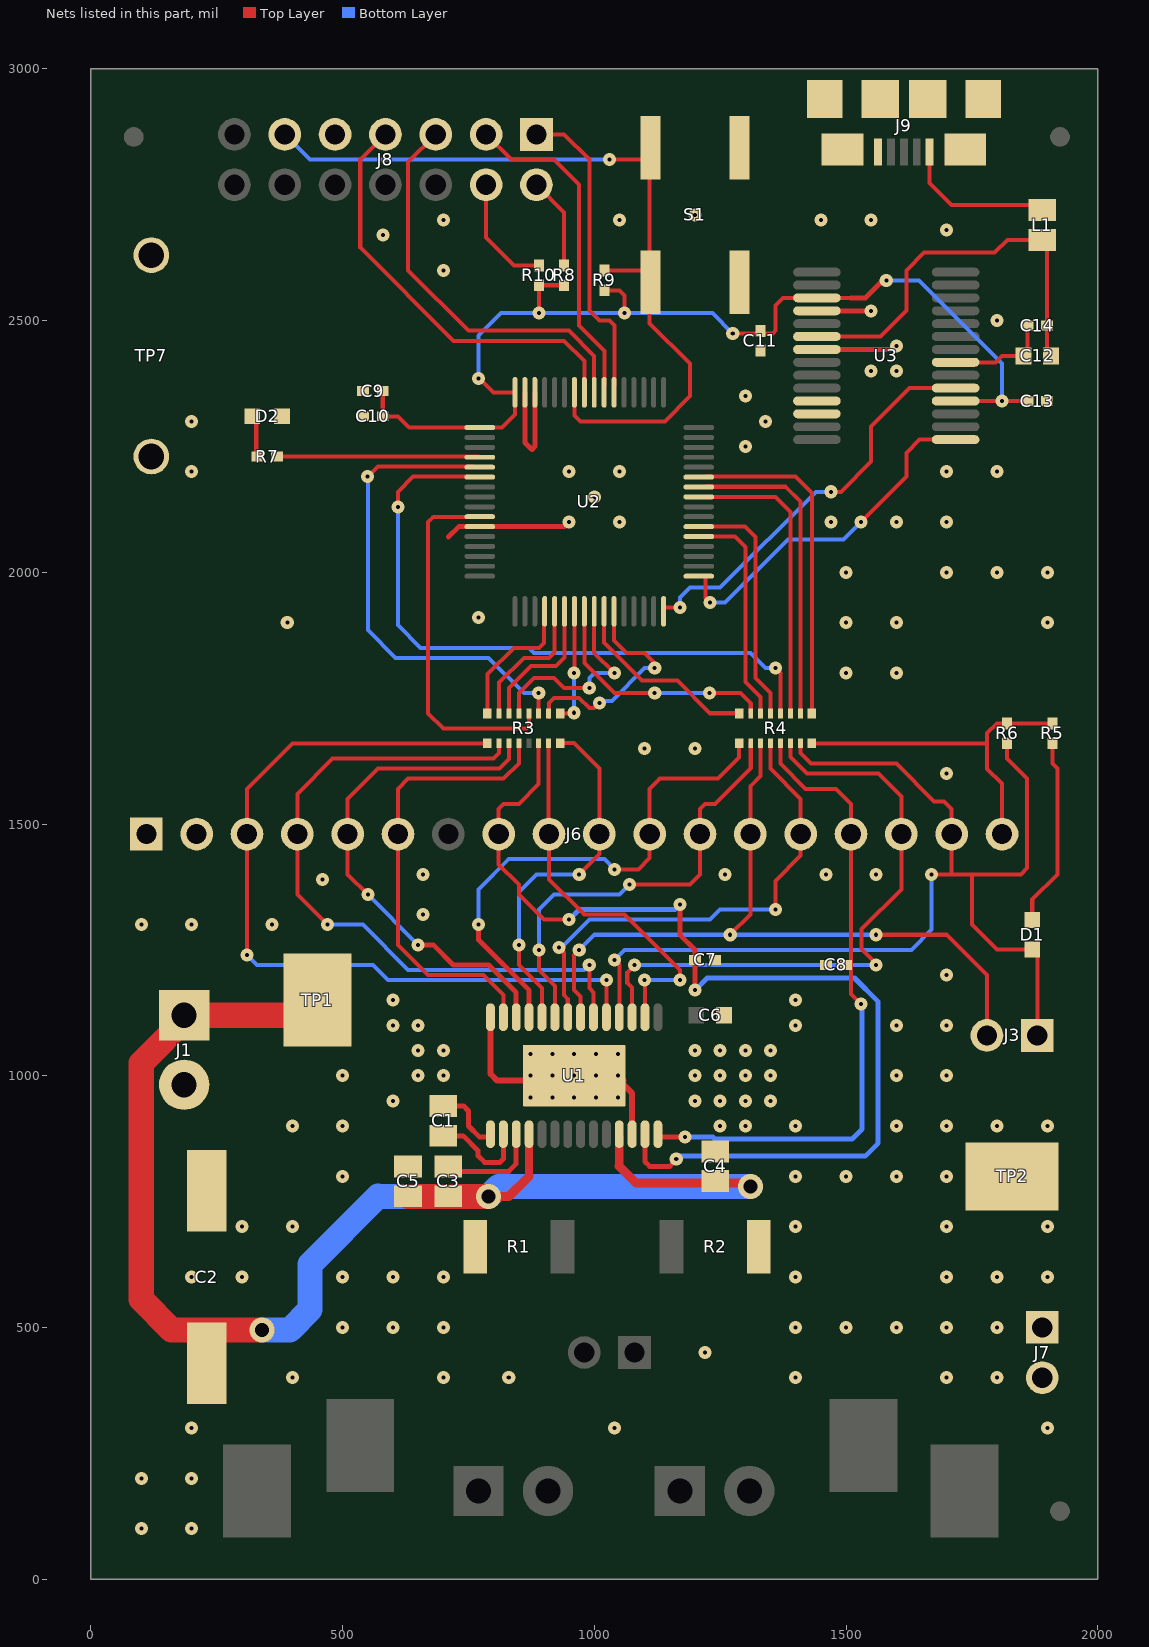
[diagram p0: the nets of this part, all layers, seen from the top]
# Altium PCB MISC86176.PcbDoc (part 2 of 2)
Units mil, origin at the board's own origin, x right, y up, seen from the top; angles counter-clockwise.
Board outline 2000 x 3000 mil, 4 copper layers (Top Layer, GND1, GND2, Bottom Layer), stack 91.4 mil thick; 53 components, 60 nets, 274 pads, 201 vias.

## Via types
v1: diameter 26, hole 8, Top Layer to Bottom Layer, tented both sides, 180 vias
v2: diameter 19.68, hole 7.87, Top Layer to Bottom Layer, 15 vias
v3: diameter 50, hole 28, Top Layer to Bottom Layer, tented both sides, 5 vias
v4: diameter 26, hole 8, Top Layer to Bottom Layer, tented top, 1 vias

## Nets (pads, with @x,y where several pads share a name; then routed paths per layer and width w, separated by ;. In a path a pad name is that pad's centre, name@x,y a point inside that pad or via, vN(x,y) a via of type N, cw(c..) or ccw(c..) an arc to the next point about the centre after c; other vN are vias at no path point) (continued)
GND: C2.2 C4.1 C5.1 C6.2 C7.2 C8.2 C9.2 C10.2 C11.2 C12.2 C13.2 C14.2 D2.2 J1.2 J6.1 J6.2 J7.1 J7.2 J8.9 J9.5 J9.6 J9.7 J9.8 J9.9 J9.10 J9.11 R1.1 R2.1 S1.1 S1.2 TP2.1 TP7.1 TP7.2 U1.12 U1.28 U1.29 U2.11 U2.62 U2.63 U3.7 U3.18 U3.21 U3.25 U3.26 | length 1423.6
  Top Layer w8: U3.7@1728.9,2417.2 1797.2,2417.2 1810,2430 C12.2@1852.44,2430 1860.31,2437.87 C14.2@1860.31,2490
  Top Layer w10: 710,2070 730.79,2090.79 U2.11@772.48,2090.79 ; U2.11@772.39,2090.7 940.7,2090.7 v1(950,2100) ; U2.63@862.05,2357.52 862.05,2257.95 876.02,2243.98 881.73,2249.69 U2.62@881.73,2357.52 ; U3.21@1430.9,2442.8 1587.2,2442.8 ; U3.18@1430.9,2519.33 U3.18@1430.9,2519.6 ; U3.18@1442.2,2519.57 1442.2,2519.33 v1(1549.33,2519.33)
  Top Layer w12: U1.28@793.66,1102.2 793.66,1003.66 807.32,990 1046.61,990 U1.29@1058.14,990 ; U1.29@1058.14,981.86 1075.16,964.84 U1.12@1075.16,883.86 U1.12@1075.16,877.8
  other v1: 100,100 200,100 100,200 200,200 200,300 1040,300 1900,300 400,400 700,400 830,400 1400,400 1700,400 1800,400 1220,450 500,500 600,500 700,500 1400,500 1500,500 1600,500 1700,500 1800,500 200,600 300,600 500,600 600,600 700,600 1400,600 1700,600 1800,600 1900,600 300,700 400,700 1400,700 1700,700 1900,700 500,800 1400,800 1500,800 1600,800 1700,800 400,900 500,900 1250,900 1300,900 1400,900 1600,900 1700,900 1800,900 1900,900 600,950 1200,950 1250,950 1300,950 1350,950 500,1000 650,1000 700,1000 1200,1000 1250,1000 1300,1000 1350,1000 1600,1000 1700,1000 650,1050 700,1050 1200,1050 1250,1050 1300,1050 1350,1050 600,1100 650,1100 1400,1100 1600,1100 1700,1100 600,1150 1400,1150 1700,1200 100,1300 200,1300 360,1300 660,1320 460,1390 660,1400 1260,1400 1460,1400 1560,1400 1700,1600 1100,1650 1200,1650 1500,1800 1600,1800 390,1900 1500,1900 1600,1900 1900,1900 770,1910 1500,2000 1700,2000 1800,2000 1900,2000 1050,2100 1470,2100 1600,2100 1700,2100 1000,2150 200,2200 950,2200 1050,2200 1700,2200 1800,2200 1300,2250 200,2300 1340,2300 1300,2350 1550,2400 1600,2400 1600,2450 1800,2500 700,2600 580,2670 1700,2680 700,2700 1050,2700 1450,2700 1550,2700 1200,2710
  other v2: 873.39,956.69 916.69,956.69 960,956.69 1003.31,956.69 1046.61,956.69 873.39,1000 916.69,1000 960,1000 1003.31,1000 1046.61,1000 873.39,1043.31 916.69,1043.31 960,1043.31 1003.31,1043.31 1046.61,1043.31
GPIO_V3P3: J6.18 R4.8 R5.2 R6.2 | length 681.8
  Top Layer w8: R4.8@1438.5,1660 1780,1660 ; J6.18@1810,1490 1810,1580 1780.31,1609.69 1780.31,1680.31 1799.69,1699.69 R6.2@1820,1699.69 R5.2@1910,1699.69
MSP_8XV3P3: R3.12 U2.10 | length 712
  Top Layer w8: U2.10@758.9,2110 680,2110 670,2100 670,1720 700,1690 865,1690 869.84,1694.84 R3.12@869.84,1719.53
MSP_ADEC_AVREF: R3.11 U2.5 | length 954.4
  Top Layer w8: v1@550,2190 570,2210 U2.5@758.9,2210 ; R3.11@889.53,1719.53 v1(889.53,1760)
  Bottom Layer w8: v1@550,2190 550,1885 605,1830 790,1830 860,1760 v1(889.53,1760) v1@890,1760
  other v1: 549.53,2190
MSP_DECAY0_ADECAY: R3.15 U2.21 | length 282.4
  Top Layer w8: R3.15@810.79,1721.5 810.79,1780.79 860,1830 867.55,1830 867.62,1830.07 910,1830.07 920.93,1841 921,1841 U2.21@921,1929
MSP_DECAY1_BDECAY: R3.16 U2.20 | length 286.3
  Top Layer w8: R3.16@787.66,1719.53 787.66,1797.66 840,1850 890,1850 900,1860 U2.20@900,1930
MSP_DIR_PHB_BIN1: R4.13 U2.38 | length 460.6
  Top Layer w8: U2.38@1220.9,2090.7 1299.3,2090.7 1320,2070 1320,1790 1350.16,1759.84 1350.16,1729.53
MSP_ENABLE_ENB_BIN2: R4.14 U2.37 | length 420.9
  Top Layer w8: U2.37@1220.9,2071 1279,2071 1300,2050 1300,1782.34 1330.47,1751.87 1330.47,1729.53
MSP_GPIO_V3P3: R4.9 U2.43 | length 653
  Top Layer w8: U2.43@1220.9,2190 1400,2190 1432.34,2157.66 1432.34,1729.53
MSP_NFAULT: R4.10 U2.42 | length 611.7
  Top Layer w8: U2.42@1220.9,2170 1380,2170 1409.21,2140.79 1409.21,1729.53
MSP_NSLEEP: R4.11 U2.41 | length 572.9
  Top Layer w8: U2.41@1220,2150 1360,2150 1390,2120 1390,1729.53
MSP_STEP_ENA_AIN2: R4.15 U2.24 | length 472.9
  Top Layer w8: U2.24@980.1,1909 980.1,1819.9 1040,1760 v1(1120,1760) ; v1(1229,1760) 1290,1760 1310.79,1739.21 R4.15@1310.79,1719.53
  Bottom Layer w8: v1(1120,1760) v1(1229,1760)
MSP_TOFF: R3.10 U2.27 | length 436.6
  Top Layer w8: R3.10@910,1712.5 910,1740 920,1750 970,1750 990,1730 1000,1730 v1(1010,1740) ; U2.27@1039.2,1909 1039.2,1864.8 1064,1840 1100,1840 1120,1820 v1(1120,1810)
  Bottom Layer w8: v1(1010,1740) 1014.8,1744.8 1034.8,1744.8 1100,1810 v1(1120,1810)
MSP_TRQ0: R3.13 U2.25 | length 400.9
  Top Layer w8: R3.13@850.16,1719.53 850.16,1760.16 880,1790 920,1790 940,1770 v1(990,1770) ; U2.25@999.8,1909 999.8,1840.2 v1(1040,1800)
  Bottom Layer w8: v1(990,1770) 990,1790 1000,1800 v1(1040,1800)
MSP_TRQ1: R3.14 U2.22 | length 284.4
  Top Layer w8: R3.14@830.47,1719.53 830.47,1770.47 874.2,1814.2 924.2,1814.2 940.7,1830.7 U2.22@940.7,1929
MSP_USM0_ADEC_PARA: R4.16 U2.26 | length 374.9
  Top Layer w8: U2.26@1019.5,1909 1019.5,1860.5 1095.13,1784.87 1165.23,1784.87 1230,1720 R4.16@1287.66,1720
MSP_USM1_PHA_AIN1: R3.9 U2.23 | length 215.4
  Top Layer w8: R3.9@932.34,1719.53 v1@959.53,1719.53 ; v1(960,1800) 960.4,1800.4 U2.23@960.4,1909
  Bottom Layer w8: v1(960,1721) v1(960,1800)
MSP_VREF_BVREF: R4.12 U2.6 | length 1287.2
  Top Layer w8: v1(610,2130) 610,2160 640,2190 U2.6@750,2190 ; v1(1359.92,1810.08) 1369.84,1800.16 1369.84,1729.53
  Bottom Layer w8: v1(610,2130) 610,1895 655,1850 870,1850 880,1840 1310.16,1840 1340.08,1810.08 v1(1359.92,1810.08)
NetC1_1: C1.1 U1.1 | length 137.2
  Top Layer w10: C1.1@700,939.53 700.47,940 740,940 750,930 750,900 772.2,877.8 U1.1@793.66,877.8
NetC1_2: C1.2 U1.2 | length 192.9
  Top Layer w10: C1.2@700,880.47 739.53,880.47 769.05,850.95 769.05,840.95 782.12,827.88 812.65,827.88 819.25,834.49 U1.2@819.25,877.8
NetD1_1: D1.1 R5.1 | length 375.6
  Top Layer w8: D1.1@1870,1309.53 1870,1350 1920,1400 1920,1610 1910,1620 R5.1@1910,1660.32
NetD2_1: D2.1 R7.1 | length 79
  Top Layer w8: R7.1@328.35,2230 D2.1@328.35,2308.99
NetJ8_2: J8.2 R8.2 | length 210.1
  Top Layer w8: J8.2@910,2770 J8.2@885,2770 940,2715 R8.2@940,2609.69 R8.2@940,2607.72
NetJ8_4: J8.4 R10.2 | length 232.5
  Top Layer w8: J8.4@785,2770 785,2665 840,2610 R10.2@889.69,2610
NFAULT: D1.2 J3.1 J6.17 R4.7 R6.1 U1.18 | length 2265.3
  Top Layer w8: v1(1040,1230) 1049.57,1220.43 U1.18@1049.57,1116.14 U1.18@1049.57,1102.2 ; R4.7@1409.21,1660.47 1409.21,1640.79 1430,1620 1600,1620 1675,1545 1695,1545 1710,1530 J6.17@1710,1480 1710,1400 ; v1(1670,1400) 1710,1400 ; R6.1@1820,1662.28 R6.1@1820,1660.32 1819.68,1630.32 1860,1590 1860,1412.2 1847.8,1400 1750,1400 ; D1.2@1870,1250.47 1799.53,1250.47 1750,1300 1750,1400 ; J3.1@1880,1080 D1.2@1880,1250 ; 1710,1400 1750,1400
  Bottom Layer w8: v1(1040,1230) 1060,1250 1630,1250 1670,1290 v1(1670,1400)
NSLEEP: J6.16 R4.6 U1.17 | length 1257.8
  Top Layer w8: U1.17@1075.16,1102.2 U1.17@1075.16,1116.14 1075.16,1174.84 1065.44,1184.56 1065.44,1205.44 v1(1080,1220) ; R4.6@1389.53,1660.47 1389.53,1632.82 1422.34,1600 1565,1600 1610,1555 J6.16@1610,1480 1610,1370 1531.22,1291.22 1531.22,1251.22 1560,1222.45 v1(1560,1220)
  Bottom Layer w8: v1@1090,1220 v1(1560,1220)
PIN13: C7.1 J6.8 R3.6 U1.13 | length 2093
  Top Layer w8: R3.6@889.53,1660.47 889.53,1579.53 850,1540 820,1540 810,1530 J6.8@810,1480 810,1420 850,1380 850,1360 900,1310 v1(950,1310)
  Top Layer w10: U1.13@1100.75,857.8 1100.75,829.25 1110,820 1150,820 1162.76,832.76 v1(1162.76,834.49) ; v1(1170,1340) 1170,1280 1200.32,1249.68 C7.1@1200.32,1230 v1(1200.32,1170)
  Bottom Layer w10: v1(950,1310) 970,1330 1160,1330 v1(1170,1340) ; v1(1162.76,834.49) 1168.27,840 1538,840 1564,866 1564,1147 1517,1194 1224.32,1194 v1(1200.32,1170)
PIN14: C8.1 J6.15 R4.5 U1.14 | length 1285.5
  Top Layer w8: R4.5@1369.84,1660.47 1369.84,1620.16 1420,1570 1480,1570 1510,1540 J6.15@1510,1480 1510,1162 v1(1530,1142)
  Top Layer w10: U1.14@1126.34,877.8 v1(1180,877.8)
  Bottom Layer w10: v1@1183.6,874.2 v1(1180,877.8) 1235.61,877.8 1239.28,874.13 1512.13,874.13 1532,894 v1@1532,1139
PIN19: J6.3 R3.1 U1.19 | length 1649.6
  Top Layer w8: v1(310,1240) J6.3@310,1480 310,1570 400,1660 R3.1@787.66,1660 ; U1.19@1023.98,1120 v1(1023.98,1190)
  Bottom Layer w8: v1(310,1240) 330,1220 560,1220 590,1190 v1(1023.98,1190)
PIN20: J6.4 R3.2 U1.20 | length 1404.4
  Top Layer w8: v1(470,1300) 410,1360 J6.4@410,1480 410,1560 480,1630 800,1630 810.79,1640.79 R3.2@810.79,1660.47 ; v1(990,1220) 990,1173.98 998.39,1165.59 998.39,1121.61 U1.20@1000,1120
  Bottom Layer w8: v1(470,1300) 540,1300 630,1210 980,1210 v1(990,1220)
PIN21: J3.2 J6.13 R4.3 U1.21 | length 1520.5
  Top Layer w8: v1(970,1250) 960,1240 960,1170 972.8,1157.2 U1.21@972.8,1120 ; v1(1270,1280) 1310,1320 J6.13@1310,1480 1310,1575 1330.47,1595.47 R4.3@1330.47,1660.47 ; v1(1560,1280) 1700,1280 1780,1200 J3.2@1780,1080
  Bottom Layer w8: v1(970,1250) 1000,1280 v1(1270,1280) v1(1560,1280)
PIN22: J6.14 R4.4 U1.22 | length 979.2
  Top Layer w8: v1(930,1255) 940,1245 940,1160 947.2,1152.8 U1.22@947.2,1120 ; R4.4@1350.16,1660.47 1350.16,1609.84 1410,1550 J6.14@1410,1480 1410,1437 1360,1387 v1(1360,1330)
  Bottom Layer w8: v1(930,1255) 935,1255 990,1310 1230,1310 1250,1330 v1(1360,1330)
PIN23: J6.12 R4.2 U1.23 | length 876
  Top Layer w8: v1(890,1250) 890,1210 921.61,1178.39 U1.23@921.61,1120 ; v1(1070,1380) 1190,1380 1210,1400 J6.12@1210,1480 1210,1530 1220,1540 1240,1540 1310.79,1610.79 R4.2@1310.79,1660.47
  Bottom Layer w8: v1@890,1260 890,1330 920,1360 1050,1360 v1(1070,1380)
PIN24: J6.10 R3.8 U1.24 | length 723.7
  Top Layer w8: v1(850,1260) 850,1220 896.02,1173.98 U1.24@896.02,1120 ; R3.8@932.34,1660.47 959.53,1660.47 1010,1610 J6.10@1010,1480 1010,1440 v4(970,1400)
  Bottom Layer w8: v1(850,1260) 850,1365 885,1400 v4(970,1400)
PIN25: J6.11 R4.1 U1.25 | length 1043.5
  Top Layer w8: v1(1040,1410) 1088,1410 1110,1432 J6.11@1110,1480 1110,1570 1130,1590 1245.32,1590 1287.66,1632.34 R4.1@1287.66,1660.47
  Top Layer w10: v1(770,1300) 770,1270 870.43,1169.57 U1.25@870.43,1120
  Bottom Layer w8: v1(770,1300) 770,1370 830,1430 1020,1430 v1(1040,1410)
RST: J8.11 R9.1 S1.3 S1.4 U2.58 | length 1740.1
  Top Layer w8: U2.58@960,2380 960.18,2357.52 U2.58@960.4,2329.6 ; U2.58@960.47,2357.52 960.47,2311.73 972.2,2300 1140,2300 1190,2350 1190,2414.72 1110,2494.72 S1.4@1110,2600 ; R9.1@1020,2600 S1.4@1110,2600 ; v1(1030,2820) S1.3@1110,2820 ; S1.3@1110,2850 S1.3@1110,2820 ; S1.4@1120,2600 S1.4@1110,2600 ; S1.3@1120,2820 S1.3@1110,2820 ; S1.4@1110,2600 S1.3@1110,2820
  Bottom Layer w8: J8.11@385,2870 435,2820 v1(1030,2820)
RX: U2.32 U3.5 | length 846
  Top Layer w8: U2.32@1137.7,1929 1138.7,1930 v1(1170,1930) ; v1(1470,2160) 1490,2160 1550,2220 1550,2290 1626,2366 U3.5@1750,2366
  Bottom Layer w8: v1(1170,1930) 1170,1950 1190,1970 1250,1970 1440,2160 v1(1470,2160)
STATUS: R7.2 U2.4 | length 398.3
  Top Layer w8: R7.2@371.65,2230 U2.4@770,2230
TCK: J8.7 U2.57 | length 832.9
  Top Layer w8: J8.7@585,2870 535,2820 535,2645 720,2460 940,2460 980.1,2419.9 U2.57@980.1,2371
TDI: J8.3 U2.55 | length 646.3
  Top Layer w8: J8.3@785,2870 834.99,2820 920,2820 970,2770 970,2490 1020,2440 1020,2371.5 U2.55@1019.5,2371
TDO: J8.1 U2.54 | length 607.5
  Top Layer w8: J8.1@885,2870 940,2870 990,2820 990,2520 1010,2500 1030,2500 1040,2490 1040,2371.8 U2.54@1039.2,2371
TMS: J8.5 U2.56 | length 791.9
  Top Layer w8: J8.5@685,2870 630,2815 630,2600 750,2480 949.6,2480 999.8,2429.8 U2.56@999.8,2371
TOFF: J6.9 R3.7 U1.16 | length 765.4
  Top Layer w8: R3.7@909.21,1660.47 909.21,1490.79 910,1490 J6.9@910,1480 910,1390 980,1320 1060,1320 1170,1210 v1(1170,1190) ; U1.16@1100.75,1120 v1@1100.75,1190
  Bottom Layer w8: v1(1100,1190) v1(1170,1190)
TRQ0: J6.6 R3.4 U1.27 | length 902.4
  Top Layer w8: U1.27@819.25,1120 819.25,1160.75 780,1200 670,1200 610,1260 J6.6@610,1480 610,1570 630,1590 820,1590 850.16,1620.16 R3.4@850.16,1660.47
TRQ1: J6.5 R3.3 U1.26 | length 1011.8
  Top Layer w8: v1(550,1360) 510,1400 J6.5@510,1480 510,1550 570,1610 811.25,1610 830.47,1629.22 R3.3@830.47,1660.47
  Top Layer w10: v1(650,1260) 680,1260 720,1220 790,1220 844.84,1165.16 U1.26@844.84,1120
  Bottom Layer w8: v1(550,1360) v1(650,1260)
TX: U2.33 U3.1 | length 762
  Top Layer w8: U2.33@1220.9,1992.2 1220.9,1949.1 v1(1230,1940) ; v1(1530,2100) 1620,2190 1620,2237.32 1646.34,2263.66 U3.1@1717.8,2263.66 ; U3.1@1693.6,2263.6 U3.1@1750,2263.6
  Bottom Layer w8: v1(1230,1940) 1260,1940 1385,2065 1495,2065 v1(1530,2100)
V3P3: C9.1 C10.1 C11.1 C13.1 R8.1 R9.2 R10.1 U2.1 U2.64 U3.4 U3.17 | length 2174.9
  Top Layer w8: C9.1@579.68,2360 C10.1@579.68,2310 610,2310 630,2290 ; 632.36,2287.64 U2.1@772.48,2287.64 816.38,2287.64 842.36,2313.62 U2.64@842.36,2357.52 799.72,2357.52 772.24,2385 v1(770,2385) ; v1(890,2515) R10.1@890,2560.32 ; R10.1@890,2570.31 R8.1@940,2570.31 ; R9.2@1020,2560.31 1020.31,2560 1050,2560 1060,2550 v1(1060,2515) ; v1(1275,2474.68) 1354.68,2474.68 1360,2480 1360,2530 1375.2,2545.2 1510,2545.2 ; U3.4@1685.4,2340.4 U3.4@1738.9,2340.4 ; U3.4@1750,2340 v1(1810,2340) C13.1@1858.37,2340
  Top Layer w10: 1510,2545.2 1538.61,2545.2 1573.41,2580 v1(1580,2580)
  Bottom Layer w8: v1@770,2380 v1(770,2385) 770,2470 815,2515 v1(890,2515) v1(1060,2515) 1234.68,2515 v1(1275,2474.68) ; v1(1580,2580) 1644.72,2580 1810,2414.72 v1(1810,2340)
VBUS: J9.1 L1.2 | length 323.2
  Top Layer w8: J9.1@1666.18,2840 J9.1@1666.18,2835 1666.18,2773.82 1710,2730 L1.2@1905,2730
VCP: C3.1 U1.3 | length 207.9
  Top Layer w10: C3.1@700,819.53 709.53,810 830,810 844.84,824.84 U1.3@844.84,877.8
VM: C2.1 C3.2 C4.2 C5.2 J1.1 TP1.1 U1.4 U1.11 | length 2972.8
  Top Layer w16: 870.43,800.43 U1.4@870.43,876.35 ; 1049.57,820.43 U1.11@1049.57,877.8
  Top Layer w18: v3@780,760 v3(790,760) 830,760 870.43,800.43 ; 1049.57,820.43 1083.31,786.69 1303.31,786.69 v3(1310,780)
  Top Layer w50: v3(340.05,495) 160.05,495 100,555.05 100,590 100,1025 195,1120 TP1.1@480,1120 ; C5.2@630,760.3 710,760.15 v3(790,760)
  Bottom Layer w50: v3(340.05,495) 395,495 435.34,535.34 435.34,625.29 570.52,760.47 v3(790,760) 810,780 v3(1310,780)
VUSB: C12.1 C14.1 L1.1 U3.20 | length 812
  Top Layer w8: U3.20@1442.2,2468.39 1568.39,2468.39 1620,2520 1620,2600 1655,2635 1795,2635 1820.47,2660.47 L1.1@1890,2660.47 1899.68,2650.79 C14.1@1899.68,2490 1899.68,2437.87 C12.1@1907.56,2430
pads on no net: FID1.1 FID2.1 FID3.1 J8.6 J8.8 J8.10 J8.12 J8.13 J8.14 J9.4 LBL1.0 U2.2 U2.3 U2.7 U2.8 U2.9 U2.12 U2.13 U2.14 U2.15 U2.16 U2.17 U2.18 U2.19 U2.28 U2.29 U2.30 U2.31 U2.34 U2.35 U2.36 U2.39 U2.40 U2.44 U2.45 U2.46 U2.47 U2.48 U2.49 U2.50 U2.51 U2.52 U2.53 U2.59 U2.60 U2.61 U3.2 U3.3 U3.6 U3.8 U3.9 U3.10 U3.11 U3.12 U3.13 U3.14 U3.19 U3.22 U3.23 U3.24 U3.27 U3.28

## Polygon pours and split planes (outlines as drawn)
GND on Top Layer "Top Layer-GND" (solid, remove dead copper, pour order 12): 0,9 0,3009 2000,3009 2000,9
GND on Bottom Layer "Bottom Layer-GND" (solid, remove dead copper, pour order 8): 0,10 0,3010 2000,3010 2000,10
GND on GND1 (split plane): 1979.9,20.1 20.1,20.1 20.1,2979.9 1979.9,2979.9
GND on GND2 (split plane): 1979.9,20.1 20.1,20.1 20.1,2979.9 1979.9,2979.9

## Keep-outs
Keep-Out Layer:
  lines w47.24: -23.62,0 ccw(c0,0) 0,-23.62 ; -23.62,0 ccw(c0,0) 0,-23.62 ; -23.62,0 -23.62,3000 ; -23.62,3000 cw(c0,3000) 0,3023.62 ; -23.62,3000 cw(c0,3000) 0,3023.62 ; 0,-23.62 2000,-23.62 ; 0,3023.62 2000,3023.62 ; 2000,-23.62 ccw(c2000,0) 2023.62,0 ; 2000,-23.62 ccw(c2000,0) 2023.62,0 ; 2000,3023.62 cw(c2000,3000) 2023.62,3000 ; 2000,3023.62 cw(c2000,3000) 2023.62,3000 ; 2023.62,0 2023.62,3000

## Other copper
Top Layer:
  region net GND: 881.73,2290 862.05,2290 862.05,2330 881.73,2330
  region net GND: 1370,2340 1520,2340 1520,2310 1370,2310
  region net GND: 805.88,1963.21 827.22,1984.55 834.55,1977.22 813.21,1955.88

## Silkscreen, mask and mechanical layers (free items; w line width, h text height)
Top Overlay:
  circle w20: c768.52,820 r8.52
  lines w7: 30,2030 720,2030 ; 120,2100 720,2100 ; 630,580 1370,580 1370,1170 1221.52,1170 ; 640,580 580,580 580,1170 1178.12,1170
  lines w8: 960,1690 1260,1690 ; 1460,1690 1680,1690
  lines w10: 120,1640 120,2170 ; 350,1640 350,2098 ; 545,1640 545,1840 ; 545,2032 545,2098 ; 30,1640 30,2170 720,2170 720,1640 30,1640
  text "MCU Reset" at 1080,2930 h30
  text "GND" at 170,2610 h40
  text "Status" at 200,2360 h30
  text "P" at 60,2126 h30
  text "DRV88XX" at 320,2125 h28
  text "I" at 60,2084 h30
  text "80" at 200,2045 h28
  text "81E" at 410,2045 h28
  text "81P" at 610,2045 h28
  text "N" at 60,2042 h30
  text "13" at 50,1980 h28
  text "ATE" at 155,1980 h28
  text "AVREF" at 480,1980 h28
  text "14" at 50,1940 h28
  text "VREF" at 155,1940 h28
  text "BVREF" at 480,1940 h28
  text "19" at 50,1900 h28
  text "DECAY1" at 155,1900 h28
  text "BDECAY" at 470,1900 h28
  text "20" at 50,1860 h28
  text "DECAY0" at 155,1860 h28
  text "ADECAY" at 470,1860 h28
  text "21" at 50,1820 h28
  text "ENABLE" at 155,1820 h28
  text "BEN" at 400,1820 h28
  text "BIN2" at 600,1820 h28
  text "22" at 50,1780 h28
  text "DIR" at 155,1780 h28
  text "BPH" at 400,1780 h28
  text "BIN1" at 600,1780 h28
  text "23" at 50,1740 h28
  text "STEP" at 155,1740 h28
  text "AEN" at 400,1740 h28
  text "AIN2" at 600,1740 h28
  text "24" at 50,1700 h28
  text "M1" at 155,1700 h28
  text "APH" at 400,1700 h28
  text "AIN1" at 600,1700 h28
  text "25" at 50,1660 h28
  text "M0" at 155,1660 h28
  text "ATE" at 395,1660 h28
  text "PARA" at 600,1660 h28
  text "GND" at 95,1410 h30 r270
  text "GND" at 190,1410 h30 r270
  text "PIN19" at 300,1410 h30 r270
  text "PIN20" at 400,1410 h30 r270
  text "TRQ1" at 500,1410 h30 r270
  text "TRQ0" at 600,1410 h30 r270
  text "8xV3P3" at 700,1410 h30 r270
  text "PIN13" at 805,1410 h30 r270
  text "TOFF" at 900,1410 h30 r270
  text "PIN24" at 995,1410 h30 r270
  text "PIN25" at 1100,1410 h30 r270
  text "PIN23" at 1200,1410 h30 r270
  text "PIN21" at 1295,1410 h30 r270
  text "PIN22" at 1395,1410 h30 r270
  text "PIN14" at 1500,1410 h30 r270
  text "nSLEEP" at 1595,1410 h30 r270
  text "nFAULT" at 1695,1410 h30 r270
  text "GPIO_V3P3" at 1790,1410 h30 r270
  text "nFAULT" at 1930,1370 h30 r270
  text "VM" at 90,1230 h40
  text "VM" at 410,980 h40
  text "Retry" at 1740,970 h40
  text "GND" at 70,840 h40
  text "GND" at 1740,660 h40
  text "Parallel" at 888,520 h45
  text "GND" at 1710,430 h40
  text "AOUT1" at 467.5,400.38 h30
  text "BOUT1" at 1470,400 h30
  text "BOUT2" at 1667.5,318.3 h30
  text "AOUT1" at 670,310 h30
  text "AOUT2" at 850,310 h30
  text "BOUT2" at 1090,310 h30
  text "BOUT1" at 1280,310 h30
  text "AOUT2" at 80,140 h30
M1 Board Outline:
  the board outline again, w10
M9 Title Sheet:
  lines w10: -491.5,5791.5 -291.5,5791.5

## Dimensions
0,3000 to 2000,0 on M2 Board Dimensions
2000,0 to 0,3000 on M2 Board Dimensions